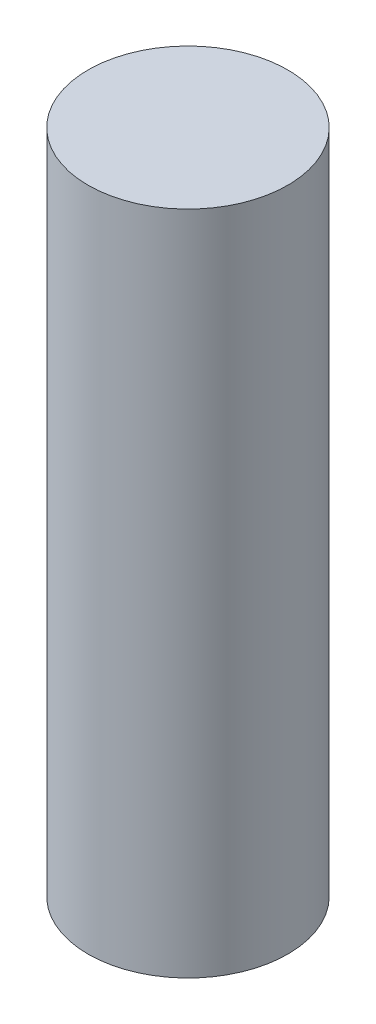
from build123d import *

# Parameters (mm, degrees)
SKETCH1_R              = 15
BOSS_EXTRUDE1_DEPTH    = 50
M20_TAPPED_HOLE1_D     = 17.5
M20_TAPPED_HOLE1_DEPTH = 62.5
M20_TAPPED_HOLE1_TIP   = 5.257530416


with BuildPart() as part:
    # Sketch1 → Boss-Extrude1 (new, symmetric)
    with BuildSketch(Plane(origin=(0, 0, 0), x_dir=(1, 0, 0), z_dir=(0, 1, 0))):
        with Locations(Location((0, 0, 0), (0, 0, 270))):
            Circle(SKETCH1_R)
    extrude(amount=BOSS_EXTRUDE1_DEPTH, both=True)

    # M20 Tapped Hole1
    with Locations(Plane(origin=(0, -50, 0), x_dir=(0, 0, -1), z_dir=(0, -1, 0))):
        with Locations((0, 0)):
            Hole(M20_TAPPED_HOLE1_D / 2, depth=M20_TAPPED_HOLE1_DEPTH)
            with Locations((0, 0, -(M20_TAPPED_HOLE1_DEPTH + M20_TAPPED_HOLE1_TIP / 2))):  # 118° drill point
                Cone(0, M20_TAPPED_HOLE1_D / 2, M20_TAPPED_HOLE1_TIP, mode=Mode.SUBTRACT)


solid = part.part
